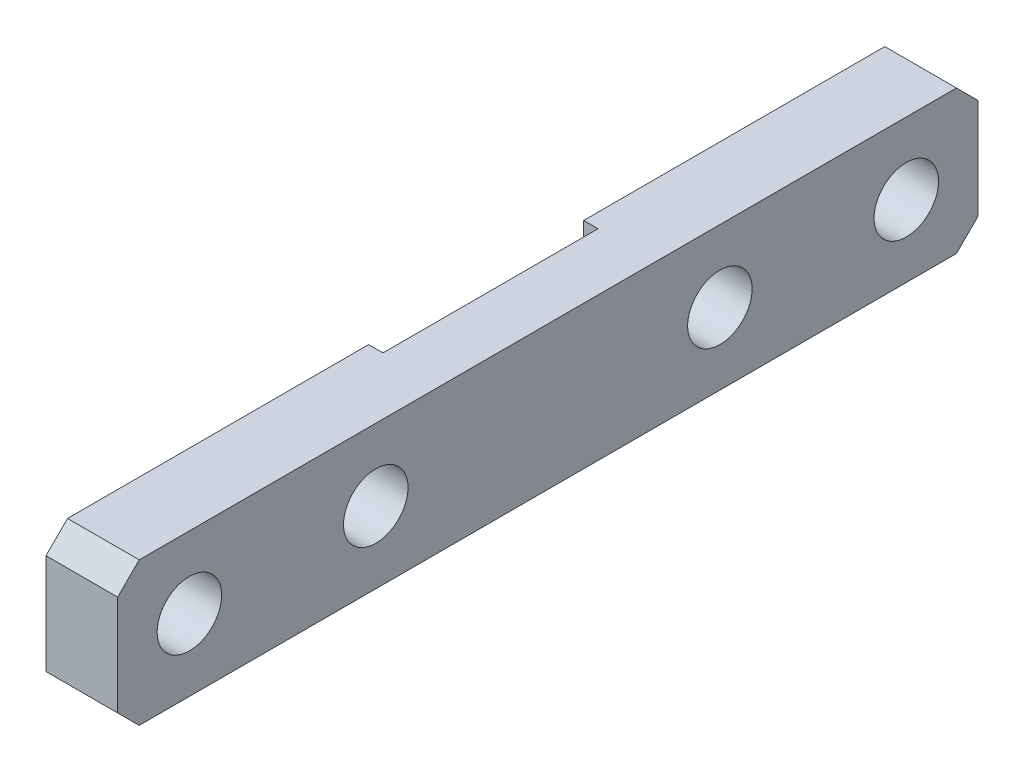
from build123d import *

# Parameters (mm, degrees)
SKETCH_1_W            = 120
SKETCH_1_H            = 20
EXTRUDE_1_DEPTH       = 10
HOLE_WIZARD_9_0_9_1_D = 9
HOLE_WIZARD_9_0_9_2_D = 9
SKETCH_6_W            = 30
SKETCH_6_H            = 20
CUT_EXTRUDE_1_DEPTH   = 2
CHAMFER_1_SIZE        = 3


with BuildPart() as part:
    # 草图1 → 凸台-拉伸1 (new body)
    with BuildSketch(Plane(origin=(0, 0, 0), x_dir=(0, 0, -1), z_dir=(1, 0, 0))):
        Rectangle(SKETCH_1_W, SKETCH_1_H)
    extrude(amount=EXTRUDE_1_DEPTH)

    # Ø9.0 (9) 直径孔1 (through all)
    with Locations(Plane(origin=(10, 0, 0), x_dir=(0, 0, -1), z_dir=(1, 0, 0))):
        with Locations((-24, 0), (24, 0)):
            Hole(HOLE_WIZARD_9_0_9_1_D / 2)

    # Ø9.0 (9) 直径孔2 (through all)
    with Locations(Plane.ZY):
        with Locations((-50, 0), (50, 0)):
            Hole(HOLE_WIZARD_9_0_9_2_D / 2)

    # 草图6 → 切除-拉伸1 (cut)
    with BuildSketch(Plane(origin=(0, 0, 0), x_dir=(0, 0, -1), z_dir=(1, 0, 0))):
        Rectangle(SKETCH_6_W, SKETCH_6_H)
    extrude(amount=CUT_EXTRUDE_1_DEPTH, mode=Mode.SUBTRACT)

    # 倒角1
    chamfer_1_edges = [part.edges().sort_by_distance(p)[0] for p in [
        (5, -10, -60),
        (5, -10, 60),
        (5, 10, 60),
        (5, 10, -60),
    ]]
    chamfer(chamfer_1_edges, length=CHAMFER_1_SIZE)


solid = part.part
